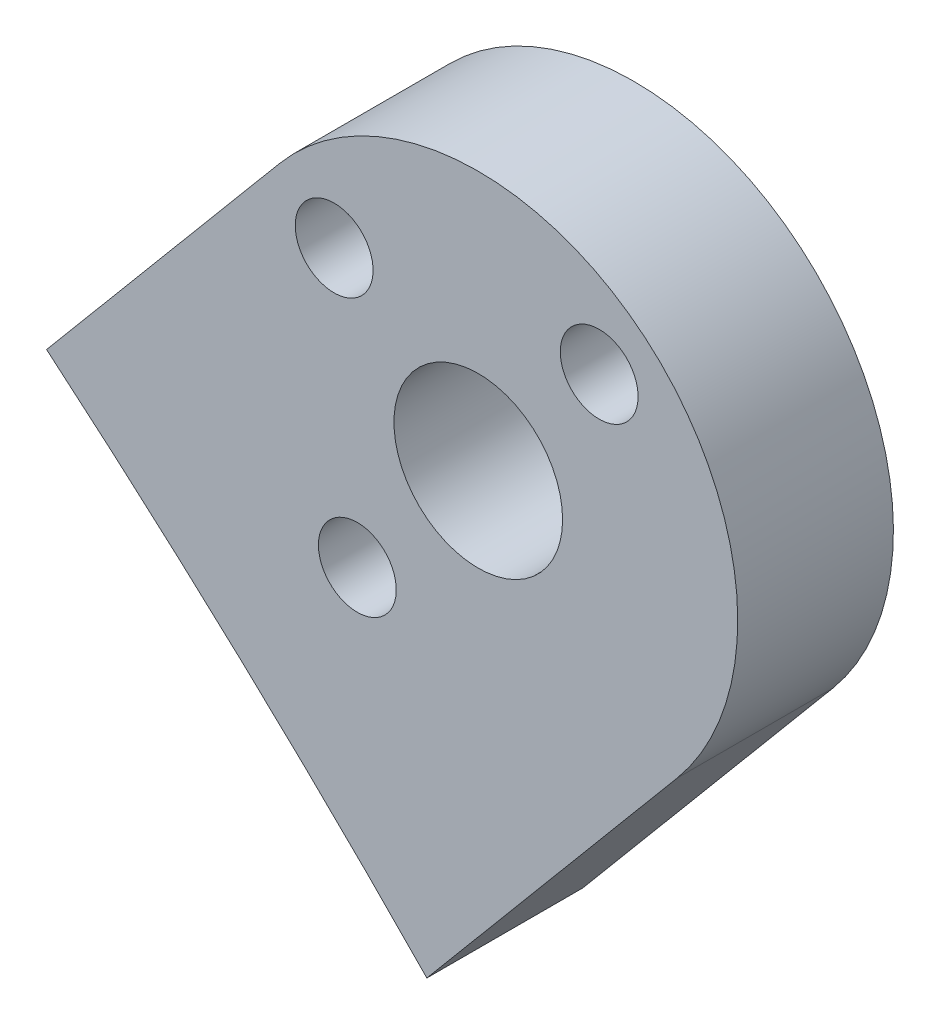
from build123d import *

# Parameters (mm, degrees)
SKETCH1_R           = 6.499999992
BOSS_EXTRUDE1_DEPTH = 6
SKETCH2_R           = 3
CUT_EXTRUDE1_DEPTH  = 12


with BuildPart() as part:
    # Sketch1 → Boss-Extrude1 (new, symmetric)
    with BuildSketch(Plane.XY):
        with BuildLine():
            Line((249.080198754, 296.842221709), (267.033227589, 318.237808321))
            ThreePointArc((267.033227589, 318.237808321), (295.209868645, 320.702944991), (297.675005315, 292.526303935))
            Line((297.675005315, 292.526303935), (278.391377025, 269.544970642))
            ThreePointArc((278.391377025, 269.544970642), (264.088717655, 283.572564272), (249.080198754, 296.842221709))
        make_face()
        with Locations((282.354116452, 305.382056128)):
            Circle(SKETCH1_R, mode=Mode.SUBTRACT)
    extrude(amount=BOSS_EXTRUDE1_DEPTH, both=True)

    # Sketch2 → Cut-Extrude1 (cut)
    with BuildSketch(Plane(origin=(0, 0, -6), x_dir=(-1, 0, 0), z_dir=(0, 0, -1))):
        with Locations(Location((-291.674536792, 316.489700554, 0), (0, 0, 90))):
            Circle(SKETCH2_R)
        with Locations(Location((-271.246472026, 314.702476468, 0), (0, 0, 90))):
            Circle(SKETCH2_R)
        with Locations(Location((-273.033696112, 294.274411702, 0), (0, 0, 90))):
            Circle(SKETCH2_R)
    extrude(amount=-CUT_EXTRUDE1_DEPTH, mode=Mode.SUBTRACT)


solid = part.part
